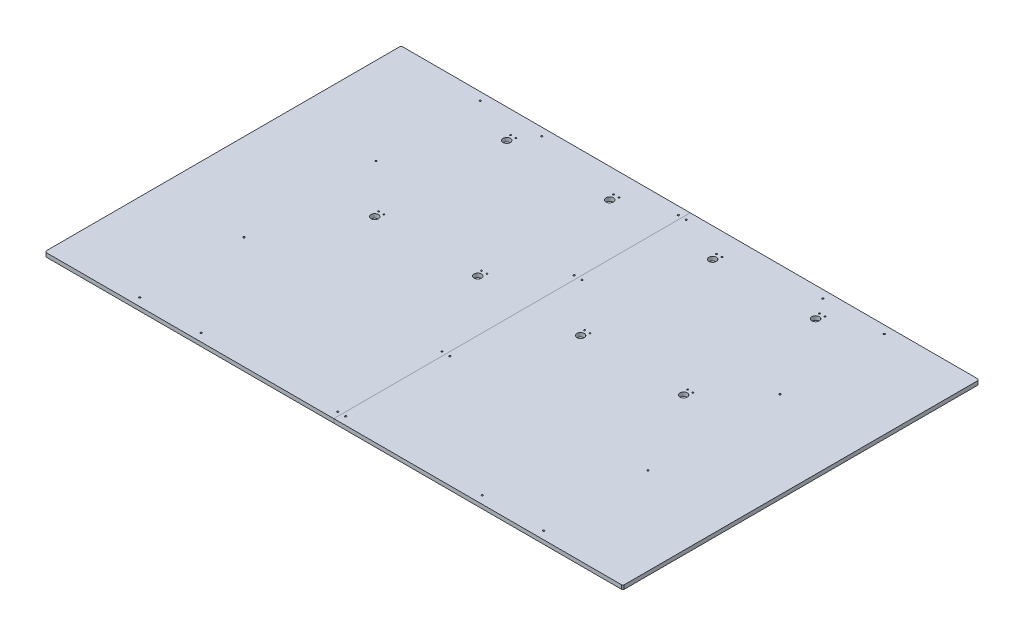
from build123d import *

# Parameters (mm, degrees)
SKETCH_1_W                = 2190
SKETCH_1_H                = 1350
EXTRUDE_1_DEPTH           = 7.5
CHAMFER_1_SIZE            = 5
HOLE_WIZARD_25_0_25_1_D   = 28
HOLE_WIZARD_2_D           = 5.5
HOLE_WIZARD_2_CBORE_D     = 10
HOLE_WIZARD_2_CBORE_DEPTH = 5.7
HOLE_WIZARD_3_D           = 6.6
HOLE_WIZARD_3_CBORE_D     = 11
HOLE_WIZARD_3_CBORE_DEPTH = 6.8


with BuildPart() as part:
    # 草图1 → 凸台-拉伸1 (new, symmetric)
    with BuildSketch(Plane(origin=(0, 0, 0), x_dir=(1, 0, 0), z_dir=(0, 1, 0))):
        Rectangle(SKETCH_1_W, SKETCH_1_H)
    extrude(amount=EXTRUDE_1_DEPTH, both=True)

    # 倒角1
    chamfer_1_edges = [part.edges().sort_by_distance(p)[0] for p in [
        (1095, 0, 675),
        (-1095, 0, 675),
        (-1095, 0, -675),
        (1095, 0, -675),
    ]]
    chamfer(chamfer_1_edges, length=CHAMFER_1_SIZE)

    # Ø25.0 (25) 直径孔1 (through all)
    with Locations(Plane(origin=(0, 7.5, 0), x_dir=(1, 0, 0), z_dir=(0, 1, 0))):
        with Locations((-585, 565), (-195, 565), (195, 565), (585, 565), (-585, 65), (-195, 65), (195, 65), (585, 65)):
            Hole(HOLE_WIZARD_25_0_25_1_D / 2)

    # 打孔尺寸(%根据)内六角圆柱头螺钉的类型2 (through all)
    with Locations(Plane.XZ.offset(7.5)):
        with Locations((-595, -590), (-575, -590), (-205, -590), (-185, -590), (185, -590), (205, -590), (575, -590), (595, -590), (-205, -90), (-185, -90), (185, -90), (205, -90), (575, -90), (595, -90), (-595, -90), (-575, -90)):
            CounterBoreHole(HOLE_WIZARD_2_D / 2, HOLE_WIZARD_2_CBORE_D / 2, HOLE_WIZARD_2_CBORE_DEPTH)

    # 打孔尺寸(%根据)内六角圆柱头螺钉的类型3 (through all)
    with Locations(Plane(origin=(0, -7.5, 0), x_dir=(-1, 0, 0), z_dir=(0, -1, 0))):
        with Locations((-765, 645), (-532.5, 645), (-765, 250), (15, 645), (15, 250), (765, 250), (532.5, 645), (765, 645), (765, -645), (532.5, -645), (765, -250), (15, -250), (15, -645), (-765, -250), (-532.5, -645), (-765, -645), (-15, -645), (-15, -250), (-15, 250), (-15, 645)):
            CounterBoreHole(HOLE_WIZARD_3_D / 2, HOLE_WIZARD_3_CBORE_D / 2, HOLE_WIZARD_3_CBORE_DEPTH)


solid = part.part
